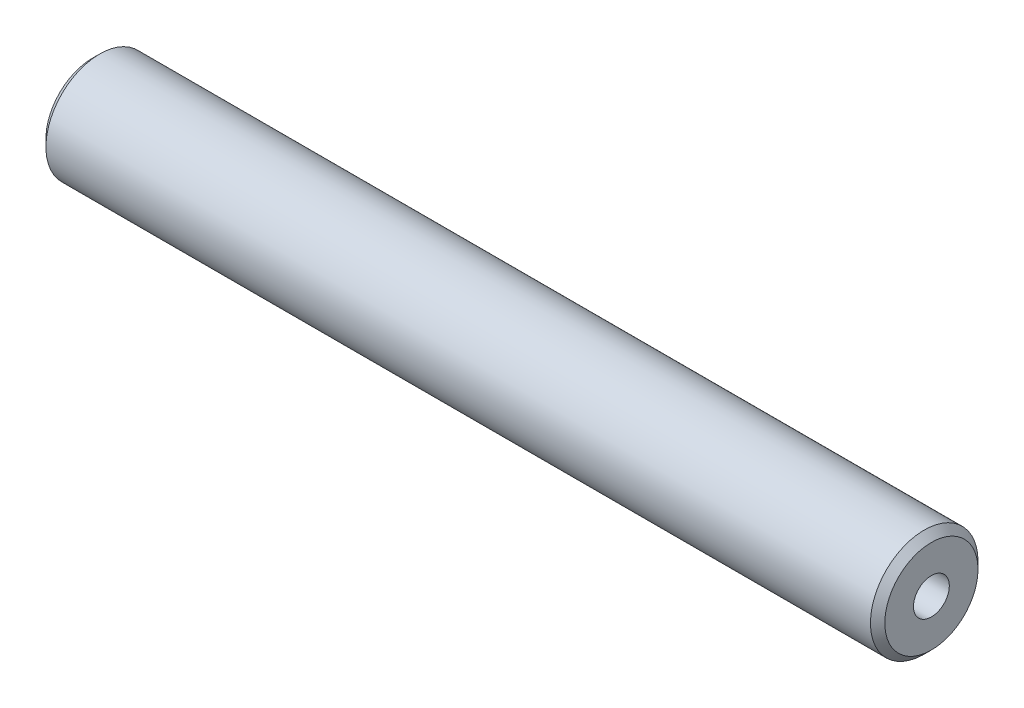
SolidWorks part; units mm, degrees
ref_plane "前视基准面" through (0, 0, 0) normal (0, 0, 1) x (1, 0, 0)
ref_plane "上视基准面" through (0, 0, 0) normal (0, 1, 0) x (1, 0, 0)
ref_plane "右视基准面" through (0, 0, 0) normal (1, 0, 0) x (0, 0, -1)
sketch "草图1" plane through (0, 0, 0) normal (1, 0, 0) x (0, 0, -1)
  circle A0 centre (0, 0) radius 7.5
  dimension "D1" = 15
extrude "凸台-拉伸1" add sketch "草图1" along normal blind 117
hole_wizard "M4 螺纹孔1" positions "草图2" profile "草图4" tap size "M4" standard "ISO"
sketch "草图2" plane through (0, 0, 0) normal (-1, 0, 0) x (0, 0, 1)
  point P0 (0, 0)
sketch "草图4" plane through (0, 0, 0) normal (0, 1, 0) x (0, 0, 1)
  line L0 (0, 0) -> (0, 11.0914)
  line L1 (0, 11.0914) -> (1.65, 10.1)
  line L2 (1.65, 10.1) -> (1.65, 0)
  line L5 (1.65, 0) -> (0, 0)
  line L10 (0, 11.0914) -> (-1.65, 10.1) construction
  line L11 (0, -6.35) -> (0, 107.95) construction
  dimension "螺纹孔钻头直径" = 3.3
  dimension "螺纹孔钻头深度" = 10.1
  dimension "导头角度" = 118
cosmetic thread "孔螺蚊线1"
hole_wizard "M6 螺纹孔1" positions "草图5" profile "草图6" tap size "M6" standard "ISO"
sketch "草图5" plane through (117, 0, 0) normal (1, 0, 0) x (0, 0, -1)
  point P0 (0, 0)
sketch "草图6" plane through (117, 0, 0) normal (0, 1, 0) x (0, 0, -1)
  line L0 (0, 0) -> (0, 16.5022)
  line L1 (0, 16.5022) -> (2.5, 15)
  line L2 (2.5, 15) -> (2.5, 0)
  line L5 (2.5, 0) -> (0, 0)
  line L10 (0, 16.5022) -> (-2.5, 15) construction
  line L11 (0, -6.35) -> (0, 107.95) construction
  dimension "螺纹孔钻头直径" = 5
  dimension "螺纹孔钻头深度" = 15
  dimension "导头角度" = 118
cosmetic thread "孔螺蚊线2" parameters "D1"=12, "D2"=6
chamfer "倒角1" distance 1 angle 45 2 edges at (0, 0, -7.5) (117, 0, -7.5)
